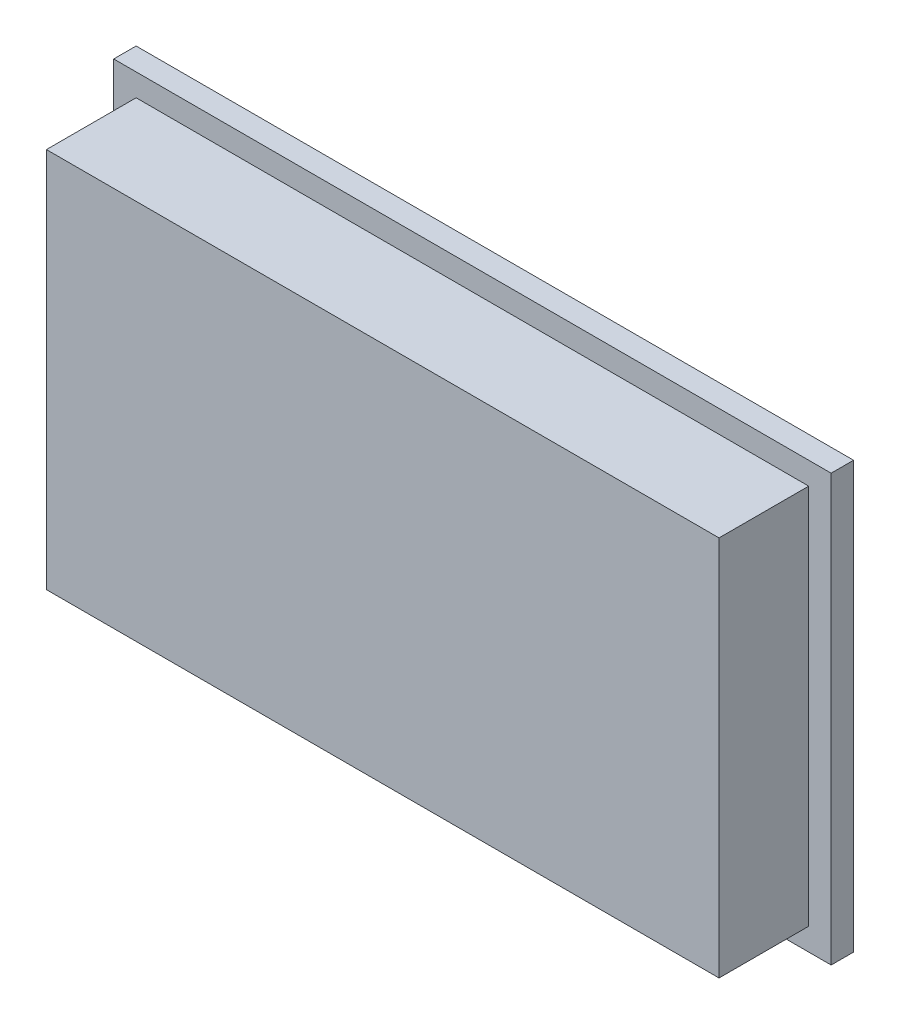
SolidWorks part; units mm, degrees
ref_plane "前视基准面" through (0, 0, 0) normal (0, 0, 1) x (1, 0, 0)
ref_plane "上视基准面" through (0, 0, 0) normal (0, 1, 0) x (1, 0, 0)
ref_plane "右视基准面" through (0, 0, 0) normal (1, 0, 0) x (0, 0, -1)
other "Configuration Table"
sketch "草图1" plane through (0, 0, 0) normal (0, 0, 1) x (1, 0, 0)
  line L0 (-32, -19) -> (32, -19)
  line L1 (32, -19) -> (32, 19)
  line L2 (32, 19) -> (-32, 19)
  line L3 (-32, 19) -> (-32, -19)
  point P0 (0, 0)
  dimension "D1" = 32
  dimension "D2" = 64
  dimension "D3" = 19
  dimension "D4" = 38
extrude "凸台-拉伸1" add sketch "草图1" against normal mid plane 2
sketch "草图2" plane through (0, 0, 0) normal (0, 0, 1) x (1, 0, 0)
  line L0 (-30, -17) -> (30, -17)
  line L1 (30, -17) -> (30, 17)
  line L2 (30, 17) -> (-30, 17)
  line L3 (-30, 17) -> (-30, -17)
  point P0 (0, 0)
  dimension "D1" = 30
  dimension "D2" = 60
  dimension "D3" = 17
  dimension "D4" = 34
extrude "凸台-拉伸2" add sketch "草图2" along normal blind 9
